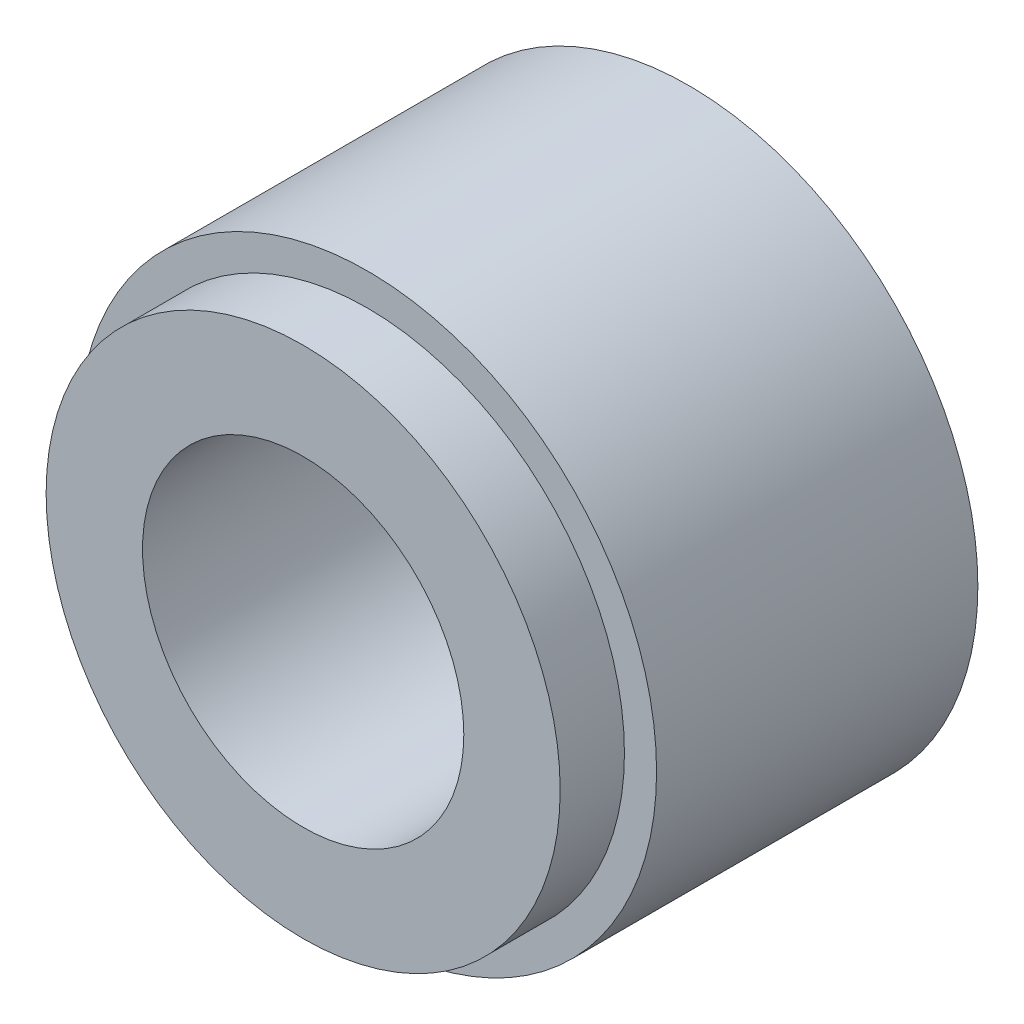
from build123d import *

# Parameters (mm, degrees)
SKETCH_1_R      = 4.5
SKETCH_1_R_2    = 2.5
EXTRUDE_1_DEPTH = 5
SKETCH_2_R      = 4
SKETCH_2_R_2    = 2.5
EXTRUDE_2_DEPTH = 1


with BuildPart() as part:
    # 草图1 → 凸台-拉伸1 (new body)
    with BuildSketch(Plane.XY):
        Circle(SKETCH_1_R)
        Circle(SKETCH_1_R_2, mode=Mode.SUBTRACT)
    extrude(amount=EXTRUDE_1_DEPTH)

    # 草图2 → 凸台-拉伸2 (add)
    with BuildSketch(Plane.XY.offset(5)):
        Circle(SKETCH_2_R)
        Circle(SKETCH_2_R_2, mode=Mode.SUBTRACT)
    extrude(amount=EXTRUDE_2_DEPTH)


solid = part.part
